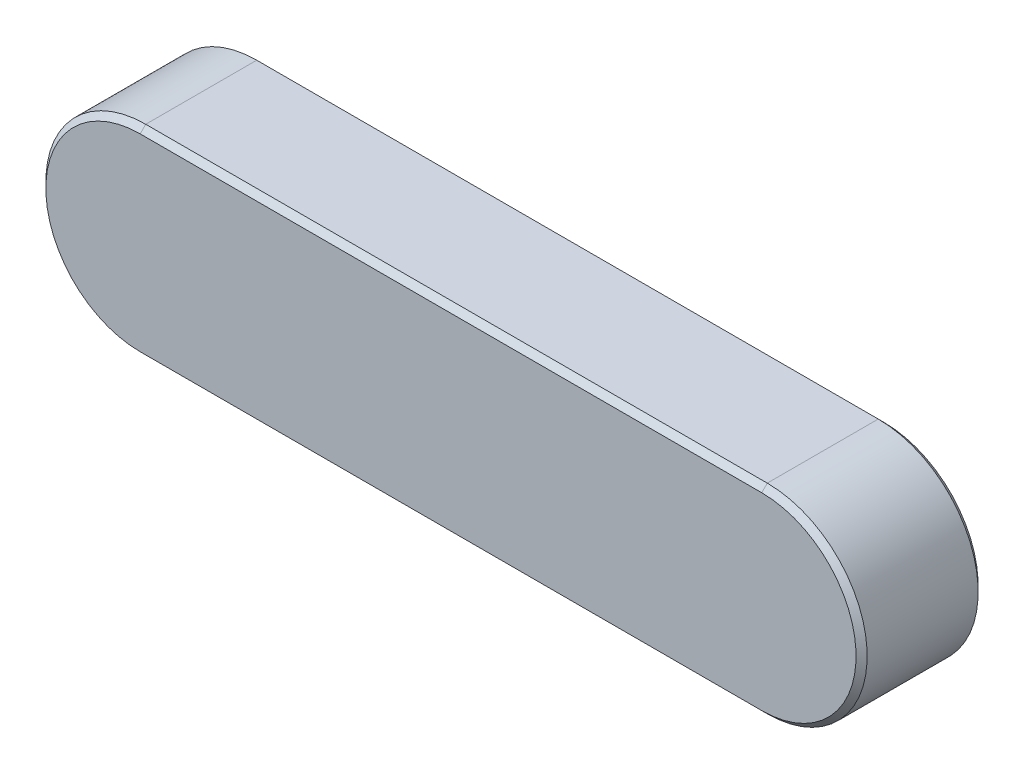
from build123d import *

# Parameters (mm, degrees)
BOSS_EXTRUDE1_DEPTH = 11
CHAMFER1_SIZE       = 0.5


with BuildPart() as part:
    # Sketch1 → Boss-Extrude1 (new body)
    with BuildSketch(Plane.XY):
        with BuildLine():
            Line((0, 9), (28, 9))
            ThreePointArc((28, 9), (37, 0), (28, -9))
            Line((28, -9), (0, -9))
            Line((0, -9), (-28, -9))
            ThreePointArc((-28, -9), (-37, 0), (-28, 9))
            Line((-28, 9), (0, 9))
        make_face()
    extrude(amount=BOSS_EXTRUDE1_DEPTH)

    # Chamfer1
    chamfer1_edges = [part.edges().sort_by_distance(p)[0] for p in [
        (0, -9, 11),
        (37, 0, 11),
        (0, 9, 11),
        (0, 9, 0),
        (37, 0, 0),
        (0, -9, 0),
        (-37, 0, 0),
        (-37, 0, 11),
    ]]
    chamfer(chamfer1_edges, length=CHAMFER1_SIZE)


solid = part.part
